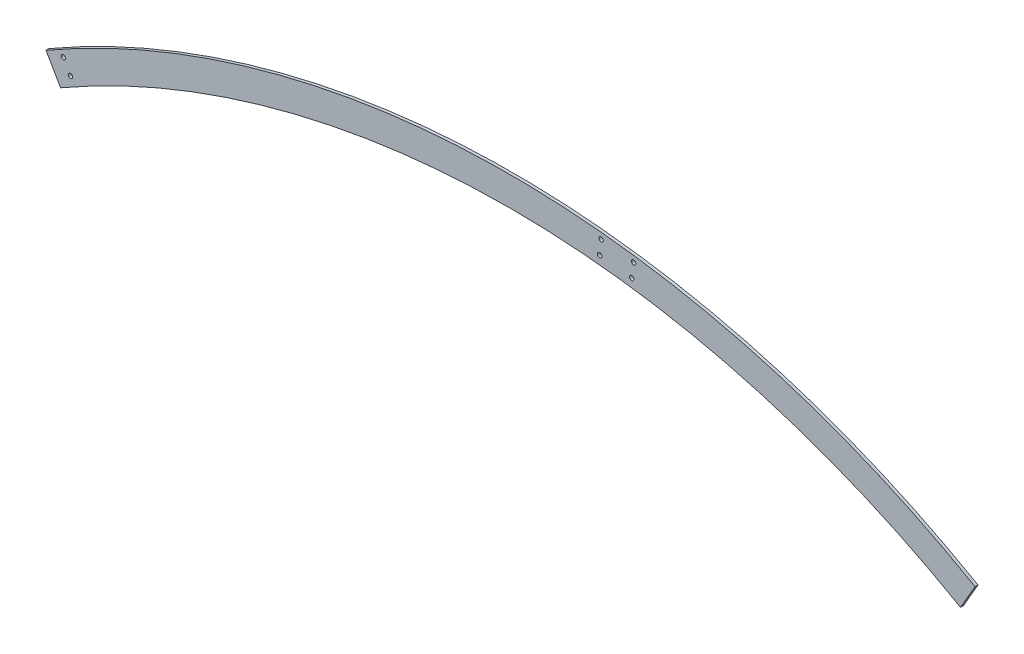
SolidWorks part; units mm, degrees
material "Q235B"
ref_plane "Front Plane" through (0, 0, 0) normal (0, 0, 1) x (1, 0, 0)
ref_plane "Top Plane" through (0, 0, 0) normal (0, 1, 0) x (1, 0, 0)
ref_plane "Right Plane" through (0, 0, 0) normal (1, 0, 0) x (0, 0, -1)
sketch "Sketch1" plane through (0, 0, 0) normal (0, 0, 1) x (1, 0, 0)
  line L0 (-1275, 69.282) -> (-1235, 0)
  line L1 (1235, 0) -> (1275, 69.282)
  line L2 (0, 410.9173) -> (0, 0) construction
  arc A0 (-1275, 69.282) -> (1275, 69.282) centre (0, -2139.0827) cw
  arc A1 (-1235, 0) -> (1235, 0) centre (0, -2139.0827) cw
  dimension "D1" = 2550
  dimension "D3" = 60
  dimension "D2" = 80
extrude "Boss-Extrude1" add sketch "Sketch1" along normal blind 8
hole_wizard "Ø12.0 (12) Diameter Hole1" positions "Sketch2" profile "Sketch3" hole size "Ø12.0" standard "GB" end condition up to next
sketch "Sketch2" plane through (0, 0, 8) normal (0, 0, 1) x (1, 0, 0)
  line L0 (0, -2139.0827) -> (-1235.5661, 91.5845) construction
  line L2 (-1275, 69.282) -> (-1235, 0) construction
  line L3 (0, -2139.0827) -> (248.4974, 381.6985) construction
  line L5 (0, -2139.0827) -> (337.8923, 371.2793) construction
  arc A0 (1235, 0) -> (-1235, 0) centre (0, -2139.0827) ccw construction
  arc A1 (1235, 0) -> (-1235, 0) centre (0, -2139.0827) ccw construction
  arc A2 (1275, 69.282) -> (-1275, 69.282) centre (0, -2139.0827) ccw construction
  circle A3 centre (0, -2139.0827) radius 2493 construction
  circle A4 centre (0, -2139.0827) radius 2533 construction
  point P0 (-1227.329, 76.7134)
  point P2 (-1207.9476, 41.7225)
  point P27 (248.4974, 381.6985)
  point P29 (244.5732, 341.8914)
  point P31 (337.8923, 371.2793)
  point P33 (332.5564, 331.6368)
  dimension "D1" = 4986
  dimension "D2" = 5066
  dimension "D5" = 35.63
  dimension "D3" = 45
  dimension "D4" = 90
sketch "Sketch3" plane through (-1227.329, 76.7134, 8) normal (1, 0, 0) x (0, -1, 0)
  line L0 (0, 0) -> (0, 8)
  line L1 (0, 8) -> (6, 8)
  line L2 (6, 8) -> (6, 0)
  line L5 (6, 0) -> (0, 0)
  line L11 (0, -6.35) -> (0, 107.95) construction
  dimension "通孔孔直径" = 12
  dimension "通孔孔深度" = 8
